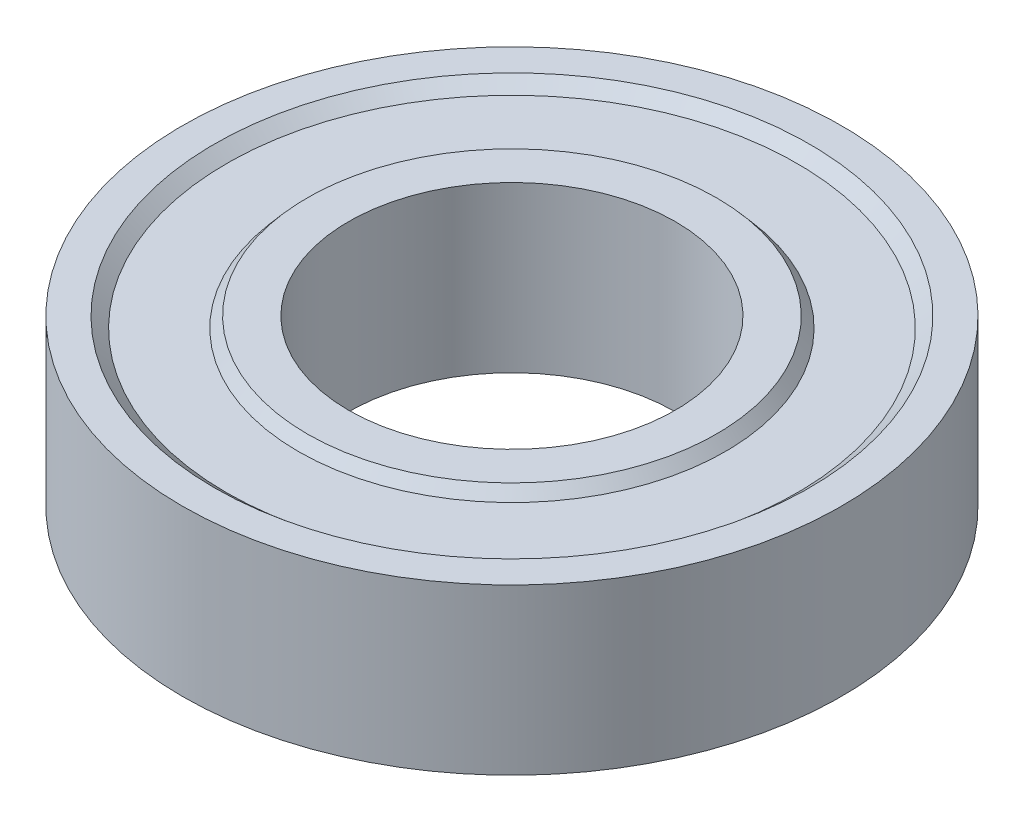
SolidWorks part; units mm, degrees
ref_plane "前视基准面" through (0, 0, 0) normal (0, 0, 1) x (1, 0, 0)
ref_plane "上视基准面" through (0, 0, 0) normal (0, 1, 0) x (1, 0, 0)
ref_plane "右视基准面" through (0, 0, 0) normal (1, 0, 0) x (0, 0, -1)
sketch "草图1" plane through (0, 0, 0) normal (0, 0, 1) x (1, 0, 0)
  line L0 (0, 19.6012) -> (0, -33.2826) construction
  line L1 (5.95, 3) -> (5.95, -3)
  line L2 (5.95, 3) -> (7.45, 3)
  line L3 (7.45, 3) -> (7.7794, 2.6141)
  line L4 (7.7794, 2.6141) -> (10.3858, 2.6141)
  line L5 (10.3858, 2.6141) -> (10.8379, 3)
  line L6 (10.8379, 3) -> (12, 3)
  line L7 (6.4568, 0) -> (4.897, 0) construction
  line L8 (10.8379, -3) -> (12, -3)
  line L9 (10.3858, -2.6141) -> (10.8379, -3)
  line L10 (7.7794, -2.6141) -> (10.3858, -2.6141)
  line L11 (7.45, -3) -> (7.7794, -2.6141)
  line L12 (5.95, -3) -> (7.45, -3)
  line L13 (12, 3) -> (12, -3)
  point P5 (5.95, 0)
  dimension "D1" = 6
  dimension "D2" = 5.95
  dimension "D3" = 1.5
  dimension "D4" = 12
revolve "旋转1" add sketch "草图1" angle 360 about L0
